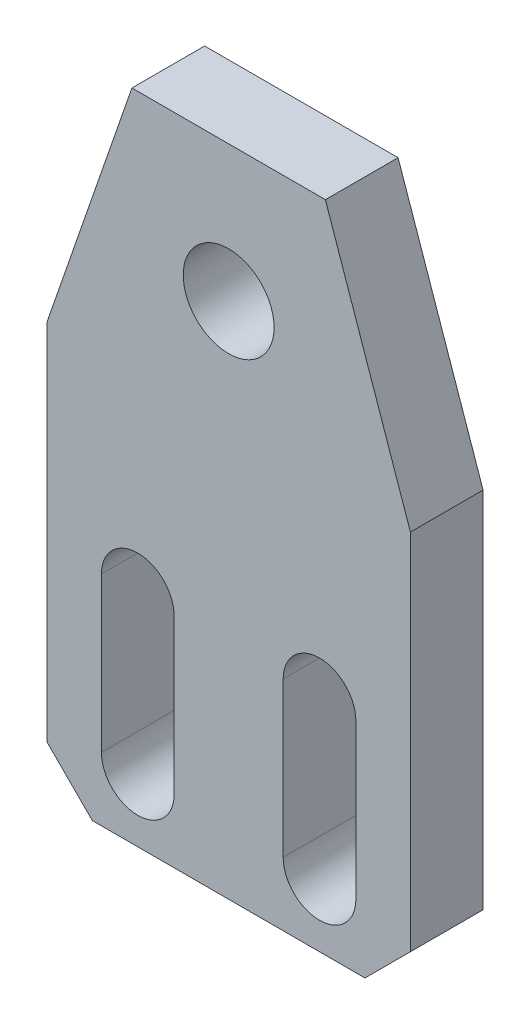
SolidWorks part; units mm, degrees
ref_plane "前视基准面" through (0, 0, 0) normal (0, 0, 1) x (1, 0, 0)
ref_plane "上视基准面" through (0, 0, 0) normal (0, 1, 0) x (1, 0, 0)
ref_plane "右视基准面" through (0, 0, 0) normal (1, 0, 0) x (0, 0, -1)
sketch "草图1" plane through (0, 0, 0) normal (0, 0, 1) x (1, 0, 0)
  line L0 (-20, 0) -> (20, 0)
  line L1 (20, 0) -> (20, 45)
  line L2 (20, 45) -> (10.6452, 72)
  line L3 (10.6452, 72) -> (-10.6452, 72)
  line L4 (-10.6452, 72) -> (-20, 45)
  line L5 (-20, 45) -> (-20, 0)
  line L6 (-20, 0) -> (-20.3226, -1.0062)
  line L7 (-14, 7) -> (-14, 24)
  line L8 (-6, 7) -> (-6, 24)
  line L9 (0, -8.0972) -> (0, 84.7441) construction
  line L10 (6, 7) -> (6, 24)
  line L11 (14, 7) -> (14, 24)
  arc A0 (-14, 7) -> (-6, 7) centre (-10, 7) ccw
  arc A1 (-6, 24) -> (-14, 24) centre (-10, 24) ccw
  arc A2 (6, 24) -> (14, 24) centre (10, 24) cw
  arc A3 (14, 7) -> (6, 7) centre (10, 7) cw
  circle A4 centre (0, 57) radius 5
  dimension "D10" = 8
  dimension "D11" = 8
  dimension "D12" = 10
  dimension "D1" = 40
  dimension "D2" = 20
  dimension "D3" = 45
  dimension "D4" = 45
  dimension "D5" = 72
  dimension "D6" = 7
  dimension "D7" = 10
  dimension "D8" = 17
  dimension "D9" = 17
  dimension "D13" = 15
extrude "凸台-拉伸1" add sketch "草图1" along normal blind 8 contours L0 L9 A4 L3 L4 L5 A1 L8 A0 L7 | L9 L0 L1 L2 L3 A4 L11 A3 L10 A2
chamfer "倒角1" distance 5 angle 45 2 edges at (-20, 0, 4) (20, 0, 4)
